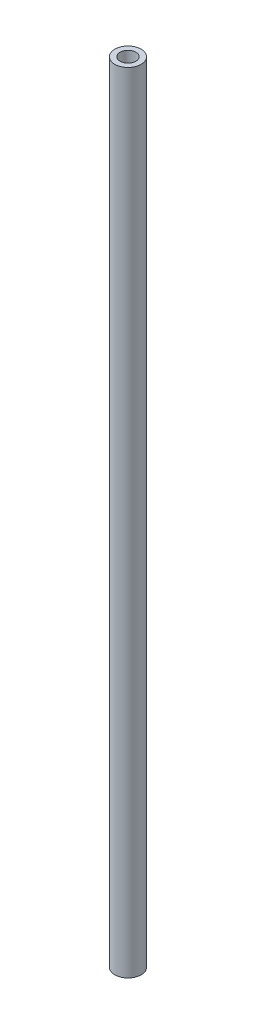
from build123d import *

# Parameters (mm, degrees)
SKETCH_1_R      = 2.5
SKETCH_1_R_2    = 1.5
EXTRUDE_1_DEPTH = 150


with BuildPart() as part:
    # 草图1 → 凸台-拉伸1 (new body)
    with BuildSketch(Plane(origin=(0, 0, 0), x_dir=(1, 0, 0), z_dir=(0, 1, 0))):
        with Locations(Location((0, 0, 0), (0, 0, 270))):
            Circle(SKETCH_1_R)
        with Locations(Location((0, 0, 0), (0, 0, 270))):
            Circle(SKETCH_1_R_2, mode=Mode.SUBTRACT)
    extrude(amount=EXTRUDE_1_DEPTH)


solid = part.part
